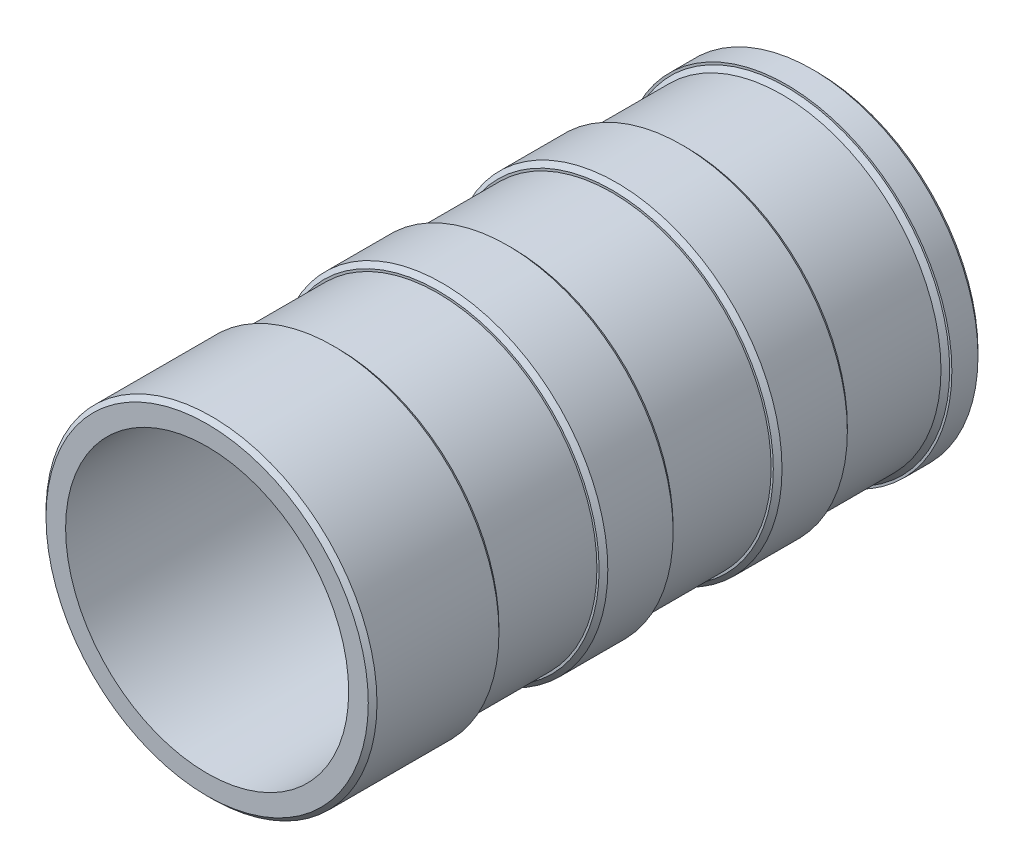
SolidWorks part; units mm, degrees
material "普通碳钢"
ref_plane "前视基准面" through (0, 0, 0) normal (0, 0, 1) x (1, 0, 0)
ref_plane "上视基准面" through (0, 0, 0) normal (0, 1, 0) x (1, 0, 0)
ref_plane "右视基准面" through (0, 0, 0) normal (1, 0, 0) x (0, 0, -1)
sketch "草图1" plane through (0, 0, 0) normal (0, 0, 1) x (1, 0, 0)
  circle A0 centre (0, 0) radius 38
  circle A1 centre (0, 0) radius 32.5
  dimension "D1" = 76
  dimension "D2" = 5.5
extrude "凸台-拉伸1" add sketch "草图1" along normal blind 140
chamfer "倒角1" distance 1 angle 45 1 edges at (38, 0, 140)
ref_plane "基准面1" through (0, 0, 110) normal (0, 0, 1) x (1, 0, 0)
sketch "草图2" plane through (0, 0, 110) normal (0, 0, 1) x (1, 0, 0)
  circle A0 centre (0, 0) radius 38
  circle A1 centre (0, 0) radius 36.5
  dimension "D1" = 76
  dimension "D2" = 73
extrude "切除-拉伸1" cut sketch "草图2" against normal blind 23
pattern_linear "阵列(线性)1" count 3 spacing 40 along (0, 0, -1) of "切除-拉伸1"
chamfer "倒角2" distance 1 angle 45 7 edges at (38, 0, 0) (36.5, 0, 7) (38, 0, 30) (38, 0, 47) (38, 0, 70) (38, 0, 87) (38, 0, 110)
